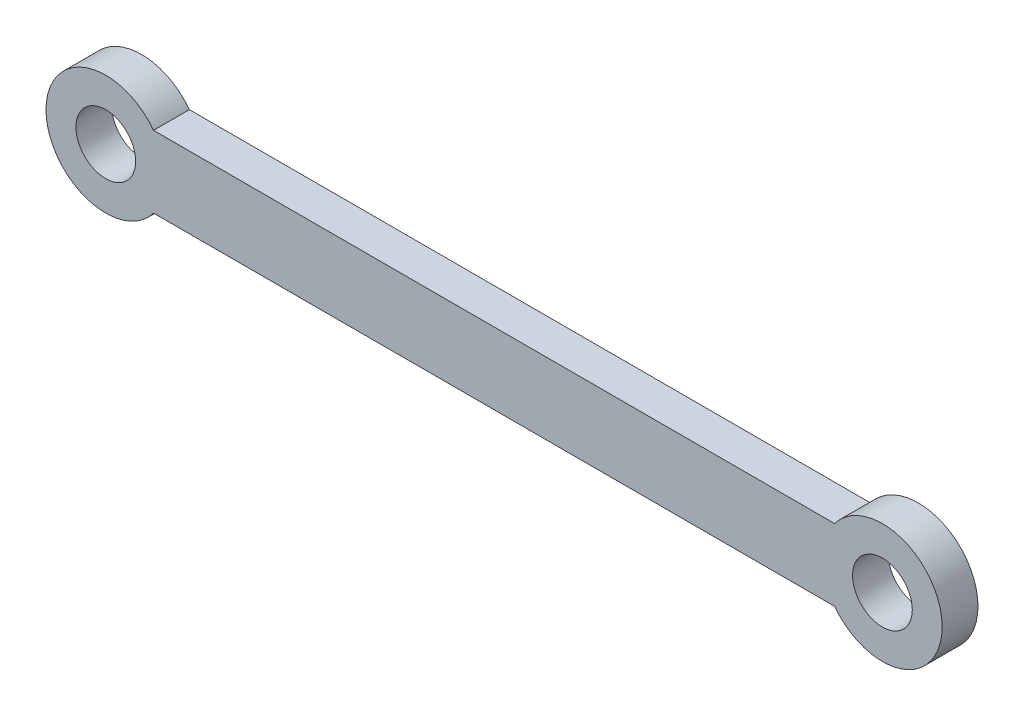
from build123d import *

# Parameters (mm, degrees)
SKETCH1_R           = 2.5
BOSS_EXTRUDE1_DEPTH = 3


with BuildPart() as part:
    # Sketch1 → Boss-Extrude1 (new body)
    with BuildSketch(Plane.XY):
        with BuildLine():
            Line((4, 3), (61, 3))
            ThreePointArc((61, 3), (70, 0), (61, -3))
            Line((61, -3), (4, -3))
            ThreePointArc((4, -3), (-5, 0), (4, 3))
        make_face()
        Circle(SKETCH1_R, mode=Mode.SUBTRACT)
        with Locations((65, 0)):
            Circle(SKETCH1_R, mode=Mode.SUBTRACT)
    extrude(amount=BOSS_EXTRUDE1_DEPTH)


solid = part.part
